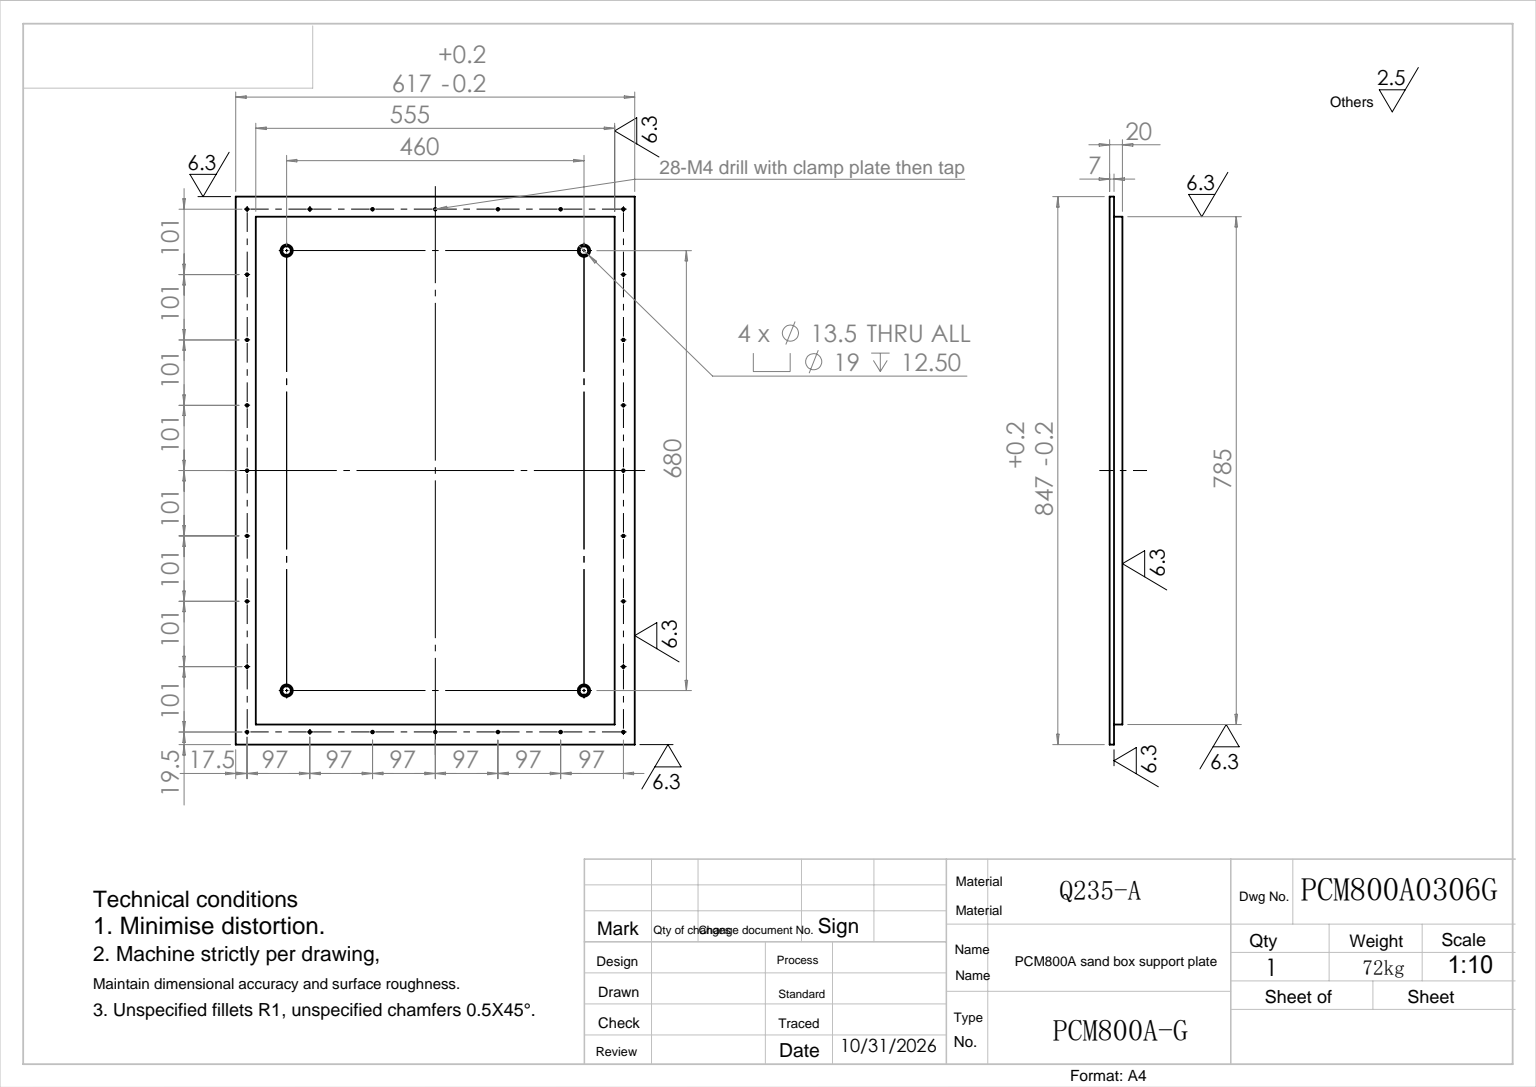
from build123d import *

# Parameters (mm, degrees)
SKETCH_1_W                    = 615
SKETCH_1_H                    = 845
EXTRUDE_1_DEPTH               = 20
SKETCH_2_W                    = 615
SKETCH_2_H                    = 30
CUT_EXTRUDE_1_DEPTH           = 13
SKETCH_3_W                    = 30
SKETCH_3_H                    = 785
CUT_EXTRUDE_2_DEPTH           = 13
HOLE_WIZARD_M4_1_D            = 4
PATTERN_LINEAR_3_COUNT        = 8
PATTERN_LINEAR_3_PITCH        = 101
PATTERN_LINEAR_4_COUNT        = 6
PATTERN_LINEAR_4_PITCH        = 97
SKETCH_15_W                   = 617
SKETCH_15_H                   = 847
SKETCH_15_W_2                 = 615
SKETCH_15_H_2                 = 845
EXTRUDE_5_DEPTH               = 7
SKETCH_17_R                   = 2.5
CUT_EXTRUDE_3_DEPTH           = 20
HOLE_WIZARD_M12_2_D           = 13.5
HOLE_WIZARD_M12_2_CBORE_D     = 19
HOLE_WIZARD_M12_2_CBORE_DEPTH = 12.5
PATTERN_LINEAR_7_COUNT        = 2
PATTERN_LINEAR_7_PITCH        = 680


with BuildPart() as part:
    # 草图1 → 拉伸1 (new body)
    with BuildSketch(Plane(origin=(0, 0, 0), x_dir=(1, 0, 0), z_dir=(0, 1, 0))):
        with Locations((307.5, 422.5)):
            Rectangle(SKETCH_1_W, SKETCH_1_H)
    extrude(amount=EXTRUDE_1_DEPTH)

    # 草图2 → 切除-拉伸1 (cut)
    with BuildSketch(Plane(origin=(0, 20, 0), x_dir=(-1, 0, 0), z_dir=(0, 1, 0))):
        with Locations((-307.5, -830)):
            Rectangle(SKETCH_2_W, SKETCH_2_H)
        with Locations((-307.5, -15)):
            Rectangle(SKETCH_2_W, SKETCH_2_H)
    extrude(amount=-CUT_EXTRUDE_1_DEPTH, mode=Mode.SUBTRACT)

    # 草图3 → 切除-拉伸2 (cut)
    with BuildSketch(Plane(origin=(0, 20, 0), x_dir=(-1, 0, 0), z_dir=(0, 1, 0))):
        with Locations((-600, -422.5)):
            Rectangle(SKETCH_3_W, SKETCH_3_H)
        with Locations((-15, -422.5)):
            Rectangle(SKETCH_3_W, SKETCH_3_H)
    extrude(amount=-CUT_EXTRUDE_2_DEPTH, mode=Mode.SUBTRACT)

    # M4 螺纹孔1 (through all)
    with Locations(Plane(origin=(598.5, 7, -826.5), x_dir=(0, 0, 1), z_dir=(0, 1, 0))):
        with Locations((0, 0), (0, -582), (808, -582), (808, 0)):
            hole_wizard_m4_1 = Hole(HOLE_WIZARD_M4_1_D / 2)

    # 阵列(线性)3: M4 螺纹孔1 ×8
    with Locations(*[(0, 0, i * PATTERN_LINEAR_3_PITCH) for i in range(1, PATTERN_LINEAR_3_COUNT)]):
        add(hole_wizard_m4_1, mode=Mode.SUBTRACT)

    # 阵列(线性)4: M4 螺纹孔1 ×6
    with Locations(*[(-i * PATTERN_LINEAR_4_PITCH, 0, 0) for i in range(1, PATTERN_LINEAR_4_COUNT)]):
        add(hole_wizard_m4_1, mode=Mode.SUBTRACT)

    # 草图15 → 凸台-拉伸5 (add)
    with BuildSketch(Plane(origin=(0, 7, 0), x_dir=(1, 0, 0), z_dir=(0, 1, 0))):
        with Locations((307.5, 422.5)):
            Rectangle(SKETCH_15_W, SKETCH_15_H)
        with Locations((307.5, 422.5)):
            Rectangle(SKETCH_15_W_2, SKETCH_15_H_2, mode=Mode.SUBTRACT)
    extrude(amount=-EXTRUDE_5_DEPTH)

    # 草图17 → 切除-拉伸3 (cut)
    with BuildSketch(Plane(origin=(0, 20, 0), x_dir=(1, 0, 0), z_dir=(0, 1, 0))):
        with Locations(Location((77.5, 82.5, 0), (0, 0, 270))):
            Circle(SKETCH_17_R)
        with Locations(Location((537.5, 82.5, 0), (0, 0, 270))):
            Circle(SKETCH_17_R)
    extrude(amount=-CUT_EXTRUDE_3_DEPTH, mode=Mode.SUBTRACT)

    # M12 六角头螺栓的柱形沉头孔2 (through all)
    with Locations(Plane(origin=(0, 20, 0), x_dir=(-1, 0, 0), z_dir=(0, 1, 0))):
        with Locations((-77.5, -82.5), (-537.5, -82.5)):
            hole_wizard_m12_2 = CounterBoreHole(HOLE_WIZARD_M12_2_D / 2, HOLE_WIZARD_M12_2_CBORE_D / 2, HOLE_WIZARD_M12_2_CBORE_DEPTH)

    # 阵列(线性)7: M12 六角头螺栓的柱形沉头孔2 ×2
    with Locations(*[(0, 0, -i * PATTERN_LINEAR_7_PITCH) for i in range(1, PATTERN_LINEAR_7_COUNT)]):
        add(hole_wizard_m12_2, mode=Mode.SUBTRACT)


solid = part.part
